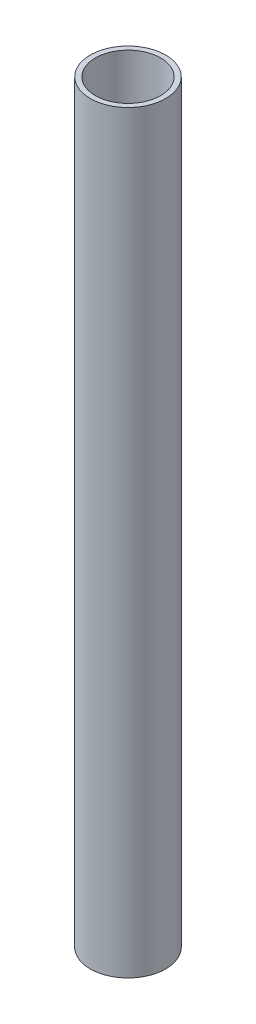
from build123d import *

# Parameters (mm, degrees)
SWEEP_THIN1_PROFILE_R   = 15
SWEEP_THIN1_PROFILE_R_2 = 13


with BuildPart() as part:
    # Sweep-Thin1: sweep along a path in Sketch1
    with BuildLine(Plane.XY) as sweep_thin1_path:
        Line((0, 0), (0, 300))
    # Sweep-Thin1 profile (on start of the path) → Sweep-Thin1 (sweep)
    with BuildSketch(Plane.ZX):
        Circle(SWEEP_THIN1_PROFILE_R)
        Circle(SWEEP_THIN1_PROFILE_R_2, mode=Mode.SUBTRACT)
    sweep(path=sweep_thin1_path.line)


solid = part.part
